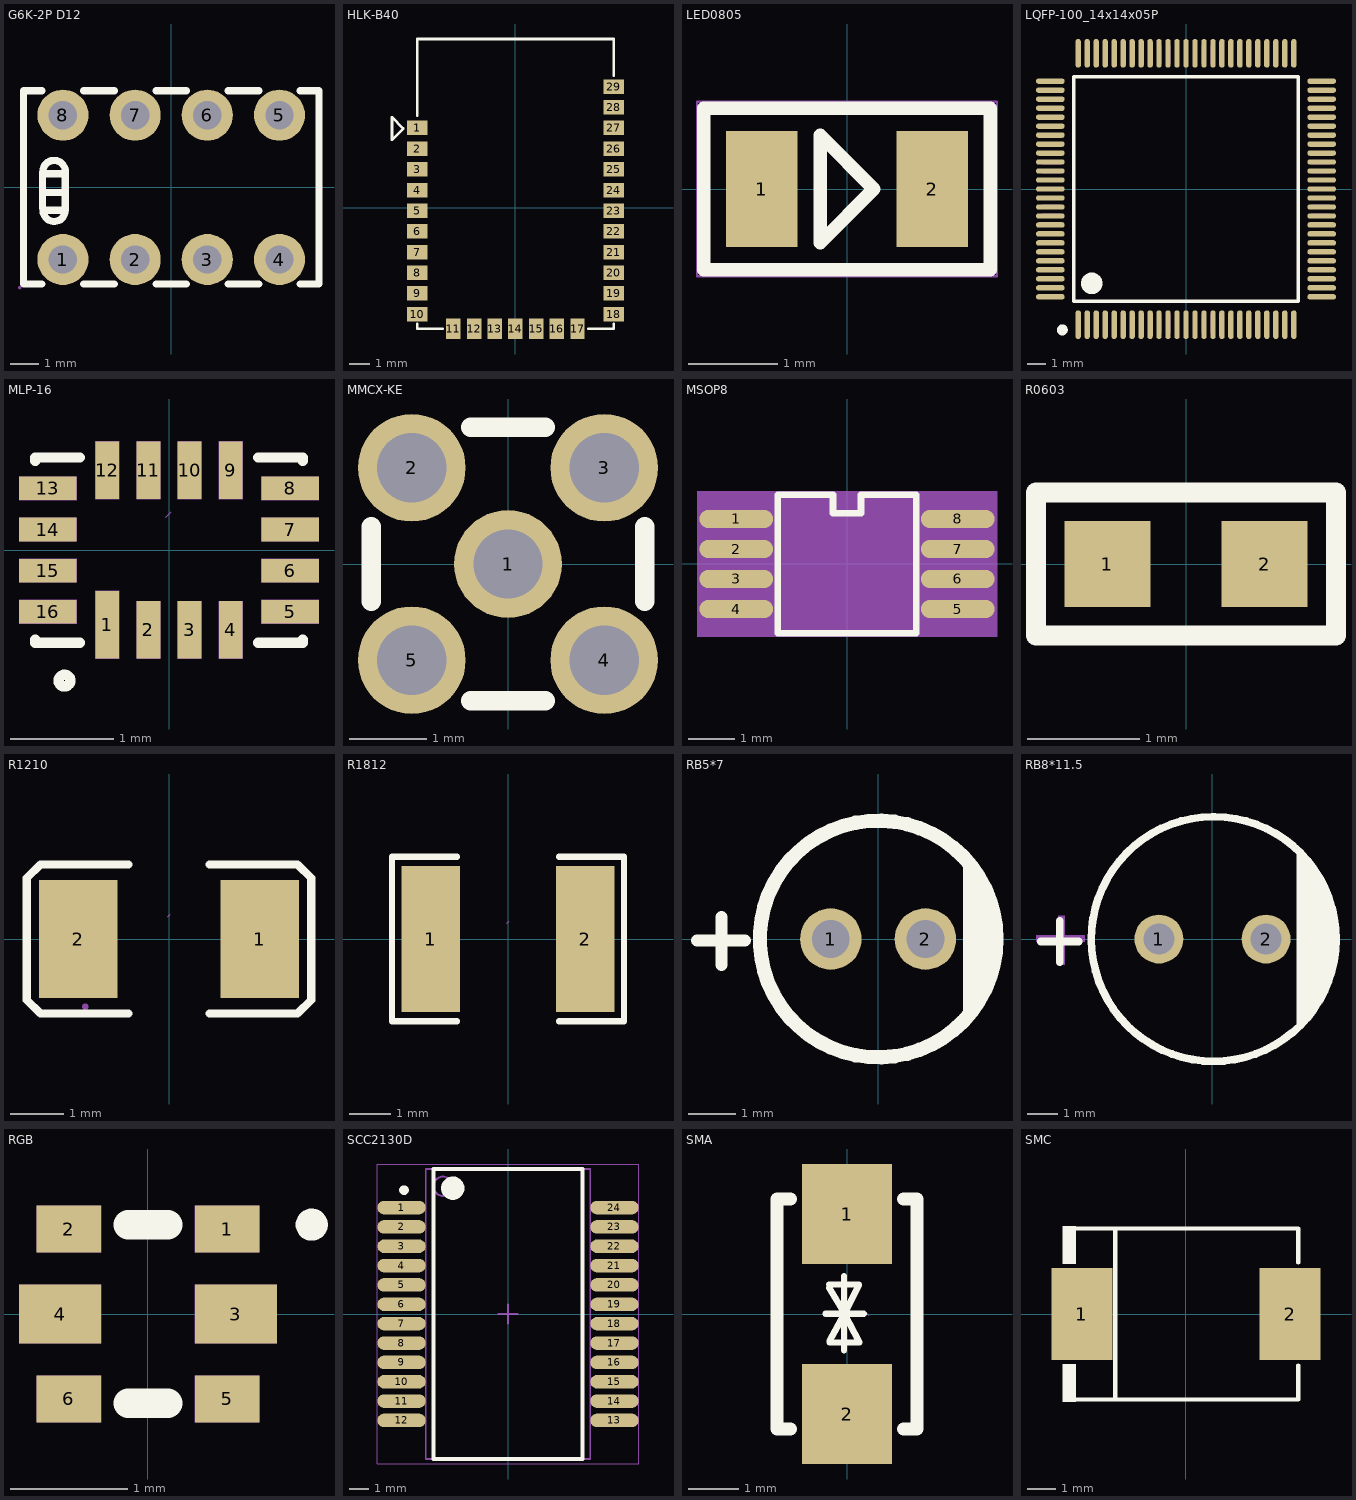
[diagram p0: the footprints below, top view; thin cyan lines are the x and y axes]
# Altium footprint library MISC84456-2.PcbLib: 53 footprints (part 2 of 4)
Each footprint in its own frame and in the unit in brackets; x right, y up, seen from the top. Pads: shape width x height; smd on the part's side, far side on the other; paste and mask are expansions set on the pad; w line width, h text height; cw(c..) or ccw(c..) is an arc to the next point about the centre after c.

## G6K-2P D12 [mm]
pads (8):
  round 1.8 hole 1: 1(-3.81,-2.54) 2(-1.27,-2.54) 3(1.27,-2.54) 4(3.81,-2.54) 5(3.81,2.54) 6(1.27,2.54) 7(-1.27,2.54) 8(-3.81,2.54)
Top Overlay:
  lines w0.254: -4.543,-3.4 -5.2,-3.4 -5.2,3.4 -4.543,3.4 ; -4.526,-0.749 -4.526,0.541 ; -4.514,0.621 cw(c-4.121,0.55) -3.729,0.48 -3.729,-0.81 ; -4.511,-0.81 ccw(c-4.121,-0.81) -3.73,-0.81 -4.51,-0.81 ; -4.51,-0.18 -3.73,-0.18 ; -4.48,0.48 -3.73,0.48 ; -3.077,-3.4 -2.003,-3.4 ; -3.077,3.4 -2.003,3.4 ; -0.537,-3.4 0.537,-3.4 ; -0.537,3.4 0.537,3.4 ; 2.003,-3.4 3.077,-3.4 ; 2.003,3.4 3.077,3.4 ; 4.543,-3.4 5.2,-3.4 5.2,3.4 4.543,3.4
Mechanical 5:
  circle w0.4: c-3.81,2.54 r0.2
  circle w0.4: c-1.27,2.54 r0.2
  circle w0.4: c1.27,2.54 r0.2
  circle w0.4: c3.81,2.54 r0.2
  circle w0.4: c3.81,-2.54 r0.2
  circle w0.4: c1.27,-2.54 r0.2
  circle w0.4: c-1.27,-2.54 r0.2
  circle w0.4: c-3.81,-2.54 r0.2
Mechanical 6:
  circle w0.06: c-5.327,-3.527 r0.03

## HLK-B40 [mm]
pads (29):
  rect 1x0.7 smd: 1(-4.75,3.85) 2(-4.75,2.85) 3(-4.75,1.85) 4(-4.75,0.85) 5(-4.75,-0.15) 6(-4.75,-1.15) 7(-4.75,-2.15) 8(-4.75,-3.15) 9(-4.75,-4.15) 10(-4.75,-5.15) 18(4.75,-5.15) 19(4.75,-4.15) 20(4.75,-3.15) 21(4.75,-2.15) 22(4.75,-1.15) 23(4.75,-0.15) 24(4.75,0.85) 25(4.75,1.85) 26(4.75,2.85) 27(4.75,3.85) 28(4.75,4.85) 29(4.75,5.85)
  rect 0.7x1 smd: 11(-3,-5.85) 12(-2,-5.85) 13(-1,-5.85) 14(0,-5.85) 15(1,-5.85) 16(2,-5.85) 17(3,-5.85)
Top Overlay:
  lines w0.127: -5.436,3.81 -5.969,3.277 -5.969,4.369 -5.436,3.835 ; -4.75,-5.613 -4.75,-5.85 -3.513,-5.85 ; -4.75,4.445 -4.75,8.128 ; -4.75,8.15 4.75,8.15 ; 3.513,-5.85 4.75,-5.85 ; 4.75,-5.613 4.75,-5.85 ; 4.75,6.376 4.75,8.15 ; 4.75,-5.85 4.75,-5.85 ; 4.75,8.15 4.75,8.15

## LED0805 [mm] "LED0805"
pads (2):
  rect 0.8x1.3 smd: 1(-0.95,0) 2(0.95,0)
Top Overlay:
  lines w0.15: -1.6,-0.9 1.6,-0.9 1.6,0.9 -0.4,0.9 -1.6,0.9 -1.6,-0.9 ; -0.3,-0.6 0.3,0 -0.3,0.6 -0.3,-0.6
Mechanical 7:
  text "1" at -1.204,0 h1.02
  text "2" at 0.696,0 h1.02
Mechanical 8:
  lines w0.025: -1.675,-0.975 -1.675,0.975 1.675,0.975 1.675,-0.975 -1.675,-0.975
Mechanical 9:
  text ".Designator" at -0.32,-0.125 h1.02
  text "GREEN" at -0.925,-0.15 h1.02

## LQFP-100_14x14x05P [mm]
pads (100):
  oval 0.3x1.6 smd: 1(-6,-7.55) 2(-5.5,-7.55) 3(-5,-7.55) 4(-4.5,-7.55) 5(-4,-7.55) 6(-3.5,-7.55) 7(-3,-7.55) 8(-2.5,-7.55) 9(-2,-7.55) 10(-1.5,-7.55) 11(-1,-7.55) 12(-0.5,-7.55) 13(0,-7.55) 14(0.5,-7.55) 15(1,-7.55) 16(1.5,-7.55) 17(2,-7.55) 18(2.5,-7.55) 19(3,-7.55) 20(3.5,-7.55) 21(4,-7.55) 22(4.5,-7.55) 23(5,-7.55) 24(5.5,-7.55) 25(6,-7.55) 51(6,7.55) 52(5.5,7.55) 53(5,7.55) 54(4.5,7.55) 55(4,7.55) 56(3.5,7.55) 57(3,7.55) 58(2.5,7.55) 59(2,7.55) 60(1.5,7.55) 61(1,7.55) 62(0.5,7.55) 63(0,7.55) 64(-0.5,7.55) 65(-1,7.55) 66(-1.5,7.55) 67(-2,7.55) 68(-2.5,7.55) 69(-3,7.55) 70(-3.5,7.55) 71(-4,7.55) 72(-4.5,7.55) 73(-5,7.55) 74(-5.5,7.55) 75(-6,7.55)
  oval 1.6x0.3 smd: 26(7.55,-6) 27(7.55,-5.5) 28(7.55,-5) 29(7.55,-4.5) 30(7.55,-4) 31(7.55,-3.5) 32(7.55,-3) 33(7.55,-2.5) 34(7.55,-2) 35(7.55,-1.5) 36(7.55,-1) 37(7.55,-0.5) 38(7.55,0) 39(7.55,0.5) 40(7.55,1) 41(7.55,1.5) 42(7.55,2) 43(7.55,2.5) 44(7.55,3) 45(7.55,3.5) 46(7.55,4) 47(7.55,4.5) 48(7.55,5) 49(7.55,5.5) 50(7.55,6) 76(-7.55,6) 77(-7.55,5.5) 78(-7.55,5) 79(-7.55,4.5) 80(-7.55,4) 81(-7.55,3.5) 82(-7.55,3) 83(-7.55,2.5) 84(-7.55,2) 85(-7.55,1.5) 86(-7.55,1) 87(-7.55,0.5) 88(-7.55,0) 89(-7.55,-0.5) 90(-7.55,-1) 91(-7.55,-1.5) 92(-7.55,-2) 93(-7.55,-2.5) 94(-7.55,-3) 95(-7.55,-3.5) 96(-7.55,-4) 97(-7.55,-4.5) 98(-7.55,-5) 99(-7.55,-5.5) 100(-7.55,-6)
Top Overlay:
  lines w0.2: -6.25,-6.25 -6.25,6.25 6.25,6.25 6.25,-6.25 -6.25,-6.25
  lines w0.3: -6.883,-7.696 ccw(c-6.882,-7.846) -6.881,-7.696
  lines w0.6: -5.25,-4.95 ccw(c-5.248,-5.25) -5.245,-4.95
Mechanical 5:
  drawing of 200 lines, arcs and shapes, not listed

## MLP-16 [mm]
pads (16):
  rect 0.23x0.66 smd: 1(-0.6,-0.726)
  rect 0.23x0.56 smd: 2(-0.2,-0.776) 3(0.2,-0.776) 4(0.6,-0.776) 9(0.6,0.776) 10(0.2,0.776) 11(-0.2,0.776) 12(-0.6,0.776)
  rect 0.56x0.23 smd: 5(1.179,-0.6) 6(1.179,-0.2) 7(1.179,0.2) 8(1.179,0.6) 13(-1.179,0.6) 14(-1.179,0.2) 15(-1.179,-0.2) 16(-1.179,-0.6)
Top Overlay:
  circle w0.1: c-1.016,-1.27 r0.057
  lines w0.1: -1.3,-0.869 -1.3,-0.9 -0.869,-0.9 ; -1.3,0.869 -1.3,0.9 -0.869,0.9 ; 0.869,-0.9 1.3,-0.9 1.3,-0.869 ; 0.869,0.9 1.3,0.9 1.3,0.869
Mechanical 5:
  region: -0.715,-0.396 -0.485,-0.396 -0.485,-1.056 -0.715,-1.056
  region: -0.315,-0.496 -0.085,-0.496 -0.085,-1.056 -0.315,-1.056
  region: 0.085,-0.496 0.315,-0.496 0.315,-1.056 0.085,-1.056
  region: 0.485,-0.496 0.715,-0.496 0.715,-1.056 0.485,-1.056
  region: 0.899,-0.485 1.459,-0.485 1.459,-0.715 0.899,-0.715
  region: 0.899,-0.085 1.459,-0.085 1.459,-0.315 0.899,-0.315
  region: 0.899,0.315 1.459,0.315 1.459,0.085 0.899,0.085
  region: 0.899,0.715 1.459,0.715 1.459,0.485 0.899,0.485
  region: -0.715,1.056 -0.485,1.056 -0.485,0.496 -0.715,0.496
  region: -0.315,1.056 -0.085,1.056 -0.085,0.496 -0.315,0.496
  region: 0.085,1.056 0.315,1.056 0.315,0.496 0.085,0.496
  region: 0.485,1.056 0.715,1.056 0.715,0.496 0.485,0.496
  region: -1.459,-0.485 -0.899,-0.485 -0.899,-0.715 -1.459,-0.715
  region: -1.459,-0.085 -0.899,-0.085 -0.899,-0.315 -1.459,-0.315
  region: -1.459,0.315 -0.899,0.315 -0.899,0.085 -1.459,0.085
  region: -1.459,0.715 -0.899,0.715 -0.899,0.485 -1.459,0.485
Mechanical 15:
  lines w0.003: -0.03,0.321 0.021,0.372

## MMCX-KE [mm]
pads (5):
  round 1.4 hole 0.9: 1(0,0) 2(-1.25,1.25) 3(1.25,1.25) 4(1.25,-1.25) 5(-1.25,-1.25)
Top Overlay:
  lines w0.254: -1.778,-0.484 -1.778,0.484 ; -0.484,-1.778 0.484,-1.778 ; -0.484,1.778 0.484,1.778 ; 1.778,-0.484 1.778,0.484
Mechanical 15:
  lines w0.003: -0.025,0.492 0.025,0.543

## MSOP8 [mil] "MSOP8"
pads (8):
  oval 63x15.7 smd: 1(-94.5,38.4) 2(-94.5,12.8) 3(-94.5,-12.8) 4(-94.5,-38.4) 5(94.5,-38.4) 6(94.5,-12.8) 7(94.5,12.8) 8(94.5,38.4)
Top Overlay:
  lines w5.9: -59.1,-59.1 59.1,-59.1 59.1,59.1 11.8,59.1 11.8,43.3 -11.8,43.3 -11.8,59.1 -59.1,59.1 -59.1,-59.1
Mechanical 7:
  text "2" at -84.5,12.8 h40
  text "1" at -84.5,38.4 h40
  text "8" at 104.5,38.4 h40
  text "6" at 104.5,-12.8 h40
  text "5" at 104.5,-38.4 h40
  text "4" at -84.5,-38.4 h40
  text "3" at -84.5,-12.8 h40
  text "7" at 104.5,12.8 h40
Mechanical 8:
  region: -128,-62 128,-62 128,62 -128,62
Mechanical 9:
  text "HYM8563" at 49.21,4.92 h40
  text ".Designator" at 31.5,-16.73 h40

## R0603 [mil]
height 43.31
pads (2):
  rect 30x30 smd: 1(-27.5,0) 2(27.5,0)
Top Overlay:
  lines w7: -52.5,-25 52.5,-25 52.5,25 -52.5,25 -52.5,-25

## R1210 [mm]
pads (2):
  rect 1.474x2.22 smd: 1(1.703,0) 2(-1.703,0)
Top Overlay:
  lines w0.152: -0.762,-1.397 -2.413,-1.397 -2.667,-1.143 -2.667,1.143 -2.413,1.397 -0.762,1.397 ; 0.762,-1.397 2.413,-1.397 2.667,-1.143 2.667,1.143 2.413,1.397 0.762,1.397
Mechanical 5:
  region: -1.6,-0.9 -1.6,0.9 -1.05,0.9 -1.05,-0.9
  region: 1.6,-0.9 1.6,0.9 1.05,0.9 1.05,-0.9
Mechanical 6:
  circle w0.06: c-1.57,-1.27 r0.03
Mechanical 15:
  lines w0.003: -0.025,0.413 0.025,0.464

## R1812 [mm]
pads (2):
  rect 1.407x3.499 smd: 1(-1.853,0) 2(1.853,0)
Top Overlay:
  lines w0.152: -1.226,-1.978 -2.785,-1.978 -2.785,1.978 -1.226,1.978 ; 1.226,-1.978 2.785,-1.978 2.785,1.978 1.226,1.978
Top Paste:
  region: -1.15,-1.65 -1.15,-0.695 -1.25,-0.595 -1.528,-0.595 -1.628,-0.495 -1.628,0.495 -1.528,0.595 -1.25,0.595 -1.15,0.695 -1.15,1.65 -1.25,1.75 -2.457,1.75 -2.557,1.65 -2.557,-1.65 -2.457,-1.75 -1.25,-1.75
  region: 1.15,-1.65 1.15,-0.695 1.25,-0.595 1.528,-0.595 1.628,-0.495 1.628,0.495 1.528,0.595 1.25,0.595 1.15,0.695 1.15,1.65 1.25,1.75 2.457,1.75 2.557,1.65 2.557,-1.65 2.457,-1.75 1.25,-1.75
Mechanical 5:
  region: 2.275,-1.62 2.275,1.62 1.525,1.62 1.525,-1.62
  region: -2.275,-1.62 -2.275,1.62 -1.525,1.62 -1.525,-1.62
Mechanical 6:
  circle w0.06: c-2.275,-1.62 r0.03
Mechanical 15:
  lines w0.003: -0.025,0.376 0.025,0.427

## RB5*7 [mm]
pads (2):
  round 1.3 hole 0.8: 1(-1,0) 2(1,0)
Top Overlay:
  circle w0.3: c0,0 r2.5
  region: 1.799,1.656 1.839,1.622 2.124,1.275 2.336,0.878 2.467,0.448 2.511,0 2.467,-0.448 2.336,-0.878 2.124,-1.275 1.839,-1.622 1.799,-1.656 1.794,-1.651
  lines w0.254: -3.826,-0.036 -2.81,-0.036 ; -3.31,-0.552 -3.31,0.464
Mechanical 5:
  circle w0.3: c-1,0 r0.15
  circle w0.3: c1,0 r0.15

## RB8*11.5 [mm]
pads (2):
  round 1.6 hole 1: 1(-1.75,0) 2(1.75,0)
Top Overlay:
  region: 2.753,-3.003 3.059,-2.654 3.375,-2.18 3.628,-1.668 3.811,-1.128 3.922,-0.569 3.959,0 3.922,0.569 3.811,1.128 3.628,1.668 3.375,2.18 3.059,2.654 2.753,3.003 2.75,3
  lines w0.254: -5.615,-0.085 -4.37,-0.085 ; -4.992,-0.758 -4.992,0.588 ; 0.003,4 ccw(c0.038,0.001) 0.074,4
Mechanical 5:
  circle w0.3: c-1.75,0 r0.15
  circle w0.3: c1.75,0 r0.15
Mechanical 15:
  region: -5.035,-0.84 -5.035,0.76 -4.835,0.76 -4.835,-0.84
  region: -5.77,0.115 -4.17,0.115 -4.17,-0.085 -5.77,-0.085

## RGB [mm]
pads (6):
  rect 0.55x0.4 smd: 1(0.675,0.725) 2(-0.675,0.725) 5(0.675,-0.725) 6(-0.675,-0.725)
  rect 0.7x0.5 smd: 3(0.75,0) 4(-0.75,0)
Top Overlay:
  circle w0.15: c1.397,0.762 r0.062
  lines w0.254: -0.169,-0.762 0.169,-0.762 ; -0.169,0.762 0.169,0.762
Mechanical 5:
  region: -0.95,-0.525 -0.4,-0.525 -0.4,-0.925 -0.95,-0.925
  region: 0.4,-0.525 0.95,-0.525 0.95,-0.925 0.4,-0.925
  region: -1.1,0.25 -0.4,0.25 -0.4,-0.25 -1.1,-0.25
  region: 0.4,0.25 1.1,0.25 1.1,-0.25 0.4,-0.25
  region: -0.95,0.925 -0.4,0.925 -0.4,0.525 -0.95,0.525
  region: 0.4,0.925 0.95,0.925 0.95,0.525 0.4,0.525

## SCC2130D [mm] "SOP, 24-Leads, Body 15.00x8.50mm, Pitch 1.00mm, IPC Medium Density"
height 4.2
pads (24):
  oval 2.5x0.7 smd: 1(-5.5,5.5) 2(-5.5,4.5) 3(-5.5,3.5) 4(-5.5,2.5) 5(-5.5,1.5) 6(-5.5,0.5) 7(-5.5,-0.5) 8(-5.5,-1.5) 9(-5.5,-2.5) 10(-5.5,-3.5) 11(-5.5,-4.5) 12(-5.5,-5.5) 13(5.5,-5.5) 14(5.5,-4.5) 15(5.5,-3.5) 16(5.5,-2.5) 17(5.5,-1.5) 18(5.5,-0.5) 19(5.5,0.5) 20(5.5,1.5) 21(5.5,2.5) 22(5.5,3.5) 23(5.5,4.5) 24(5.5,5.5)
Top Overlay:
  circle w0.6: c-2.85,6.5 r0.3
  circle w0.25: c-5.375,6.4 r0.125
  lines w0.2: -3.85,-7.5 3.85,-7.5 3.85,7.5 -3.85,7.5 -3.85,-7.5
Mechanical 13:
  circle w0.1: c-3.35,6.6 r0.5
  lines w0.1: -4.25,-7.5 4.25,-7.5 4.25,7.5 -4.25,7.5 -4.25,-7.5
Mechanical 15:
  lines w0.05: -6.75,-7.75 6.75,-7.75 6.75,7.75 -6.75,7.75 -6.75,-7.75
  lines w0.1: -0.5,0 0.5,0 ; 0,-0.5 0,0.5
3D body: height 4.2, standoff 0.25, extent -4.25,-7.5 4.25,7.5

## SMA [mm]
pads (2):
  rect 1.8x2 smd: 1(0,2) 2(0,-2)
Top Overlay:
  lines w0.127: -0.43,0.002 -0.049,0.002 ; -0.36,0.53 -0.049,0.002 ; -0.36,0.59 0.24,0.59 -0.049,0.002 ; -0.35,-0.57 0.25,-0.57 -0.049,0.002 ; -0.35,-0.54 -0.049,0.002 ; -0.06,-0.73 -0.06,0.76 ; 0.332,0.002 -0.049,0.002
  lines w0.254: -1.131,-2.3 -1.4,-2.3 -1.4,2.3 -1.131,2.3 ; 1.131,-2.3 1.4,-2.3 1.4,2.3 1.131,2.3
Mechanical 15:
  lines w0.003: 0.386,0.025 0.437,-0.025

## SMC [mm]
pads (2):
  rect 2.158x3.24 smd: 1(-3.686,0) 2(3.686,0)
Top Overlay:
  region: -3.9,3.102 -3.9,1.772 -4.357,1.772 -4.357,3.102
  region: -3.9,-3.102 -3.9,-1.772 -4.357,-1.772 -4.357,-3.102
  lines w0.152: -3.976,-3.026 3.976,-3.026 3.976,-1.823 ; -3.976,3.026 3.976,3.026 3.976,1.823 ; -2.504,-3.026 -2.504,3.026
Mechanical 5:
  region: -3.95,-1.5 -3.95,1.5 -2.7,1.5 -2.7,-1.5
Mechanical 6:
  circle w0.06: c-4.13,-2.95 r0.03